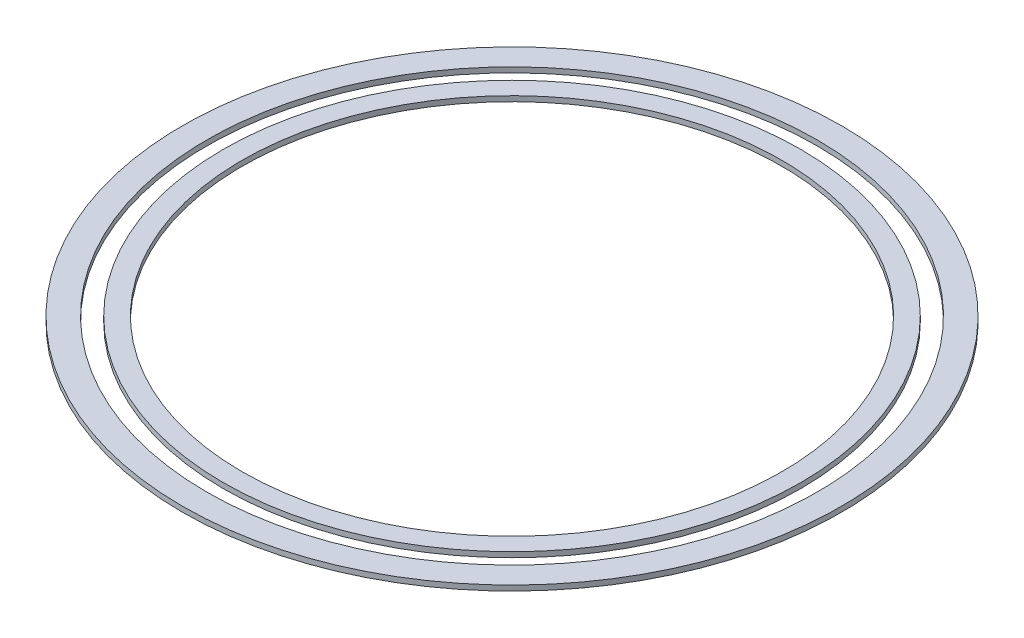
SolidWorks part; units mm, degrees
ref_plane "Front Plane" through (0, 0, 0) normal (0, 0, 1) x (1, 0, 0)
ref_plane "Top Plane" through (0, 0, 0) normal (0, 1, 0) x (1, 0, 0)
ref_plane "Right Plane" through (0, 0, 0) normal (1, 0, 0) x (0, 0, -1)
sketch "Sketch1" plane through (0, 0, 0) normal (0, 0, 1) x (1, 0, 0)
  line L0 (0, 0) -> (0, -12.063) construction
  line L2 (74.4957, 137.5) -> (68.9708, 137.5)
  line L3 (74.4957, 137.5) -> (74.4957, 136.3145)
  line L4 (74.4957, 136.3145) -> (68.9708, 136.3145)
  line L5 (68.9708, 137.5) -> (68.9708, 136.3145)
  line L6 (-60.9957, 137.5) -> (60.9957, 137.5) construction
  line L7 (60.9957, 137.5) -> (65.2618, 137.5)
  line L8 (60.9957, 137.5) -> (60.9957, 136.3145)
  line L9 (60.9957, 136.3145) -> (65.2618, 136.3145)
  line L10 (65.2618, 137.5) -> (65.2618, 136.3145)
  line L11 (-63.9957, 137.5) -> (63.9957, 137.5) construction
revolve "Revolve1" add sketch "Sketch1" angle 360 about L0
